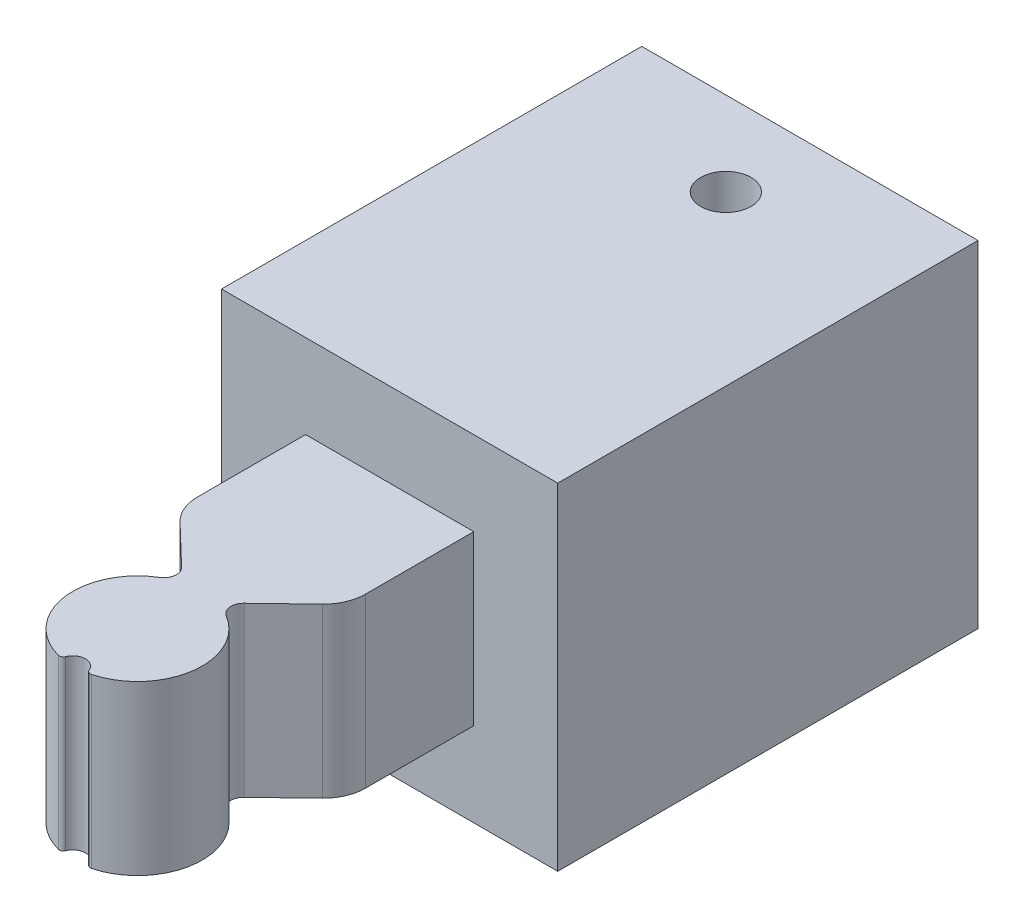
from build123d import *

# Parameters (mm, degrees)
BOSS_EXTRUDE1_DEPTH = 20
SKETCH2_W           = 40
SKETCH2_H           = 50
BOSS_EXTRUDE2_DEPTH = 10
SKETCH3_W           = 40
SKETCH3_H           = 50
BOSS_EXTRUDE3_DEPTH = 10
SKETCH4_R           = 3
CUT_EXTRUDE1_DEPTH  = 59


with BuildPart() as part:
    # Sketch1 → Boss-Extrude1 (new body)
    with BuildSketch(Plane(origin=(0, 0, 0), x_dir=(1, 0, 0), z_dir=(0, 1, 0))):
        with BuildLine():
            Line((8.463180042, -41.475773732), (3.711045987, -46.039141468))
            ThreePointArc((3.711045987, -46.039141468), (3.259281785, -47.287683344), (3.975543478, -48.405680168))
            ThreePointArc((3.975543478, -48.405680168), (7.623740011, -56.081012602), (1.985598103, -62.439583333))
            ThreePointArc((1.985598103, -62.439583333), (1.632656794, -62.403507094), (1.392497371, -62.14237013))
            ThreePointArc((1.392497371, -62.14237013), (0, -61.2), (-1.392497371, -62.14237013))
            ThreePointArc((-1.392497371, -62.14237013), (-1.632656794, -62.403507094), (-1.985598103, -62.439583333))
            ThreePointArc((-1.985598103, -62.439583333), (-7.623740011, -56.081012602), (-3.975543478, -48.405680168))
            ThreePointArc((-3.975543478, -48.405680168), (-3.259281785, -47.287683344), (-3.711045987, -46.039141468))
            Line((-3.711045987, -46.039141468), (-8.463180042, -41.475773732))
            ThreePointArc((-8.463180042, -41.475773732), (-9.59977718, -39.82945203), (-10, -37.869337265))
            Line((-10, -37.869337265), (-10, -25))
            Line((-10, -25), (-20, -25))
            Line((-20, -25), (-20, 25))
            Line((-20, 25), (20, 25))
            Line((20, 25), (20, -25))
            Line((20, -25), (10, -25))
            Line((10, -25), (10, -37.869337265))
            ThreePointArc((10, -37.869337265), (9.59977718, -39.82945203), (8.463180042, -41.475773732))
        make_face()
    extrude(amount=BOSS_EXTRUDE1_DEPTH)

    # Sketch2 → Boss-Extrude2 (add)
    with BuildSketch(Plane(origin=(0, 20, 0), x_dir=(1, 0, 0), z_dir=(0, 1, 0))):
        Rectangle(SKETCH2_W, SKETCH2_H)
    extrude(amount=BOSS_EXTRUDE2_DEPTH)

    # Sketch3 → Boss-Extrude3 (add)
    with BuildSketch(Plane.XZ):
        Rectangle(SKETCH3_W, SKETCH3_H)
    extrude(amount=BOSS_EXTRUDE3_DEPTH)

    # Sketch4 → Cut-Extrude1 (cut)
    with BuildSketch(Plane.XZ.offset(10)):
        with Locations(Location((0, -15, 0), (0, 0, 270))):
            Circle(SKETCH4_R)
    extrude(amount=-CUT_EXTRUDE1_DEPTH, mode=Mode.SUBTRACT)


solid = part.part
